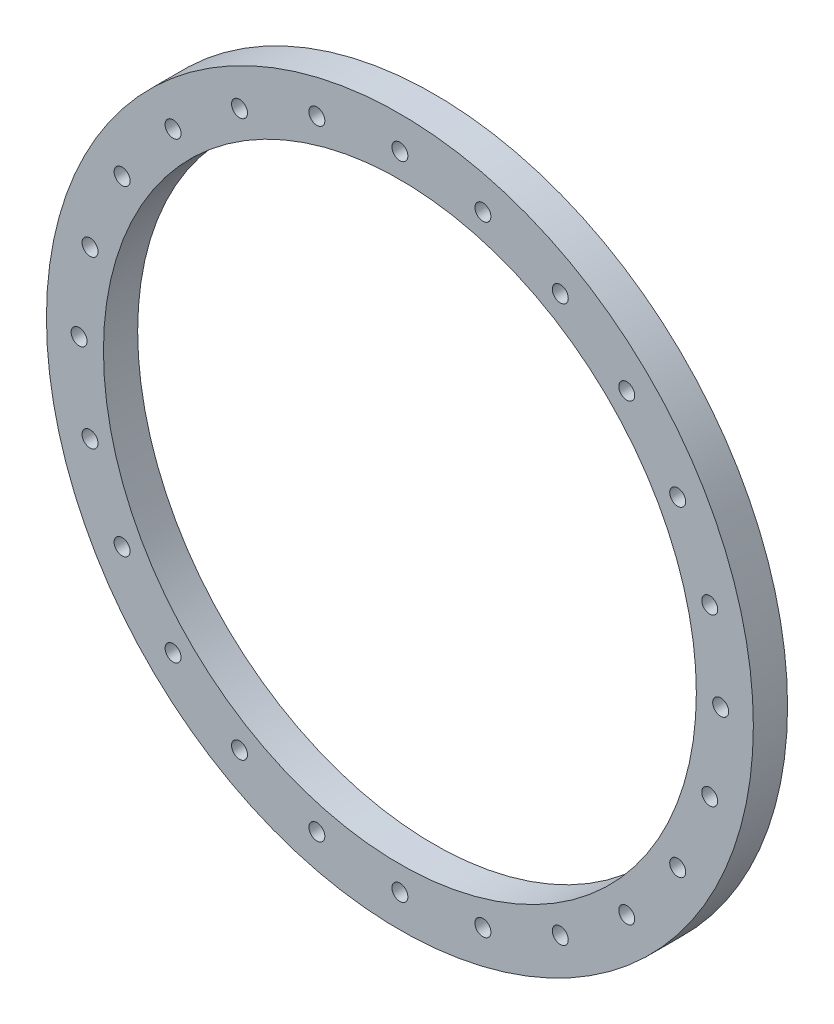
SolidWorks part; units mm, degrees
material "Q235"
ref_plane "Front Plane" through (0, 0, 0) normal (0, 0, 1) x (1, 0, 0)
ref_plane "Top Plane" through (0, 0, 0) normal (0, 1, 0) x (1, 0, 0)
ref_plane "Right Plane" through (0, 0, 0) normal (1, 0, 0) x (0, 0, -1)
sketch "Sketch1" plane through (0, 0, 0) normal (0, 0, 1) x (1, 0, 0)
  circle A0 centre (0, 0) radius 465
  circle A1 centre (0, 0) radius 390
  dimension "D1" = 930
  dimension "D2" = 780
extrude "Boss-Extrude1" add sketch "Sketch1" along normal blind 45
sketch "Sketch2" plane through (0, 0, 45) normal (0, 0, 1) x (1, 0, 0)
  line L0 (-465, 0) -> (465, 0) construction
  circle A0 centre (0, 0) radius 422 construction
  circle A1 centre (0, 0) radius 465 construction
  dimension "D1" = 844
hole_wizard "M24 Threaded hole1" positions "3DSketch1" profile "Sketch3" tap size "M24" standard "GB" end condition through all
sketch3d "3DSketch1"
  line L0 (-465, 0, 45) -> (465, 0, 45) construction
  circle A0 centre (0, 0, 45) radius 422 construction
  point P0 (-422, 0, 45)
  point P6 (0, 0, 467)
sketch "Sketch3" plane through (-422, 0, 45) normal (1, 0, 0) x (0, -1, 0)
  line L0 (0, 0) -> (0, 45)
  line L1 (0, 45) -> (10.5, 45)
  line L2 (10.5, 45) -> (10.5, 0)
  line L5 (10.5, 0) -> (0, 0)
  line L11 (0, -6.35) -> (0, 107.95) construction
  dimension "通孔螺纹孔钻头直径" = 21
  dimension "通孔螺纹孔钻头深度" = 45
cosmetic thread "孔螺蚊线1" parameters "D2"=24
pattern_circular "Circular pattern1" count 24 every 15 about axis through (0, 0, 0) along (0, 0, 1) of "M24 Threaded hole1"
